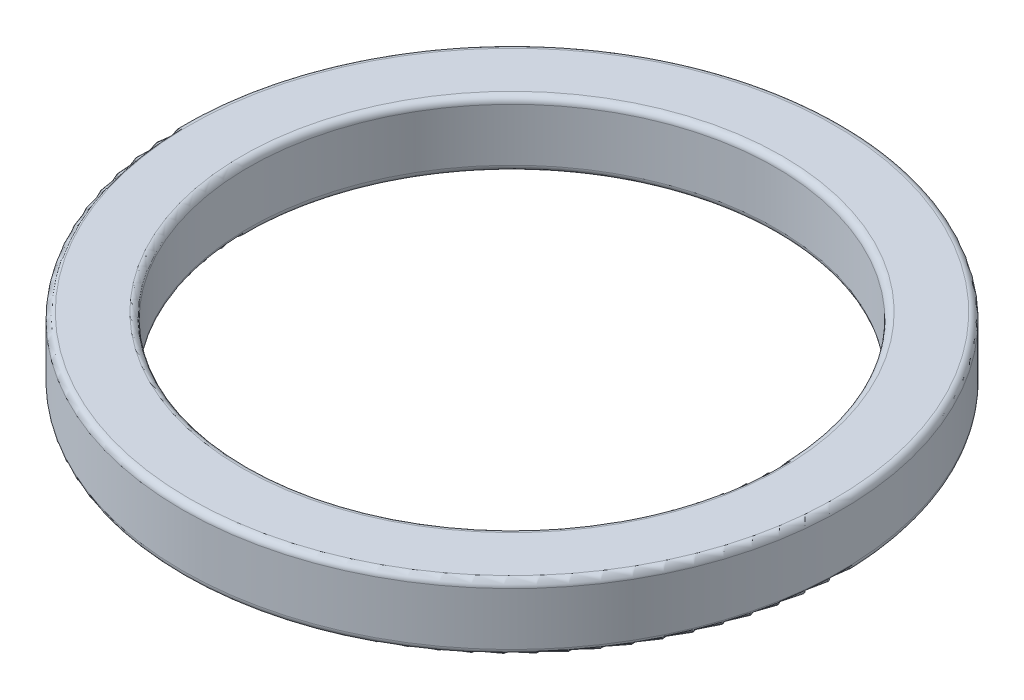
SolidWorks part; units mm, degrees
material "标准件"
ref_plane "前视基准面" through (0, 0, 0) normal (0, 0, 1) x (1, 0, 0)
ref_plane "上视基准面" through (0, 0, 0) normal (0, 1, 0) x (1, 0, 0)
ref_plane "右视基准面" through (0, 0, 0) normal (1, 0, 0) x (0, 0, -1)
sketch "草图1" plane through (0, 0, 0) normal (0, 1, 0) x (1, 0, 0)
  circle A0 centre (0, 0) radius 40
  circle A1 centre (0, 0) radius 50
  dimension "D1" = 100
  dimension "D2" = 80
extrude "凸台-拉伸1" add sketch "草图1" along normal blind 10
fillet "圆角1" radius 1 4 edges at (0, 0, 50) (0, 10, 50) (0, 0, 40) (0, 10, 40)
